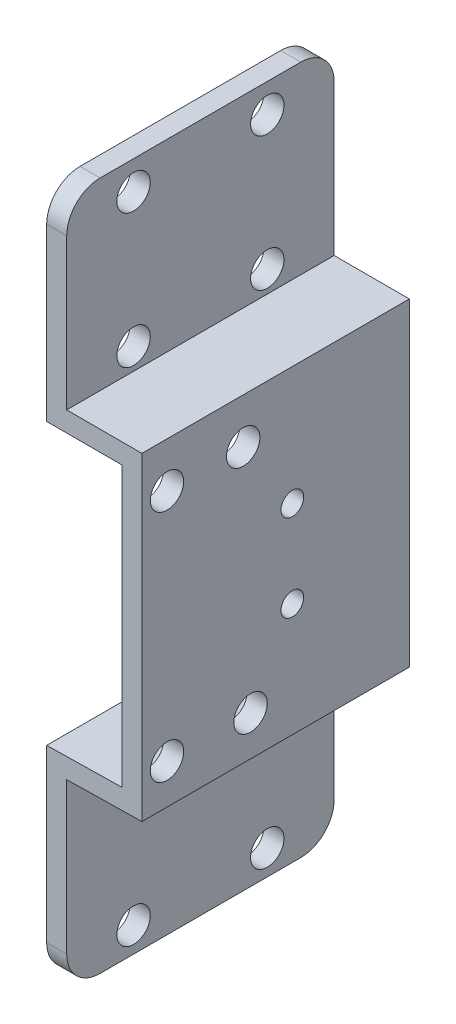
from build123d import *

# Parameters (mm, degrees)
EXTRUDE_THIN1_DEPTH   = 20
FILLET1_R             = 5
SIZE_MM_DOWEL_HOLE1_D = 5
M4_TAPPED_HOLE1_D     = 3.4


with BuildPart() as part:
    # Sketch1 → Extrude-Thin1 (new, symmetric)
    with BuildSketch(Plane.XY):
        Polygon((-5.625, 51.525), (-5.625, 20.975), (5.625, 20.975), (5.625, -20.777349891), (-5.625, -20.974615696), (-5.625, -51.525), (-2.625, -51.525), (-2.625, -23.922472646), (8.625, -23.725206841), (8.625, 23.975), (-2.625, 23.975), (-2.625, 51.525), align=None)
    extrude(amount=EXTRUDE_THIN1_DEPTH, both=True)

    # Fillet1
    fillet1_edges = [part.edges().sort_by_distance(p)[0] for p in [
        (-4.125, 51.525, -20),
        (-4.125, -51.525, -20),
        (-4.125, 51.525, 20),
        (-4.125, -51.525, 20),
    ]]
    fillet(fillet1_edges, radius=FILLET1_R)

    # Size mm Dowel Hole1 (through all)
    with Locations(Plane(origin=(8.625, 0, 0), x_dir=(0, 0, -1), z_dir=(1, 0, 0))):
        with Locations((-3.75, -17.768125), (-16.25, -17.768125), (-4.858090708, 17.231875), (-16.25, 17.231875), (10, 47.231875), (10, 27.231875), (-10, 27.231875), (-10, 47.231875), (10, -47.768125), (10, -27.768125), (-10, -27.768125), (-10, -47.768125)):
            Hole(SIZE_MM_DOWEL_HOLE1_D / 2)

    # M4 Tapped Hole1 (through all)
    with Locations(Plane(origin=(8.625, 0, 0), x_dir=(0, 0, -1), z_dir=(1, 0, 0))):
        with Locations((2.5, -6.768125), (2.5, 6.231875)):
            Hole(M4_TAPPED_HOLE1_D / 2)


solid = part.part
